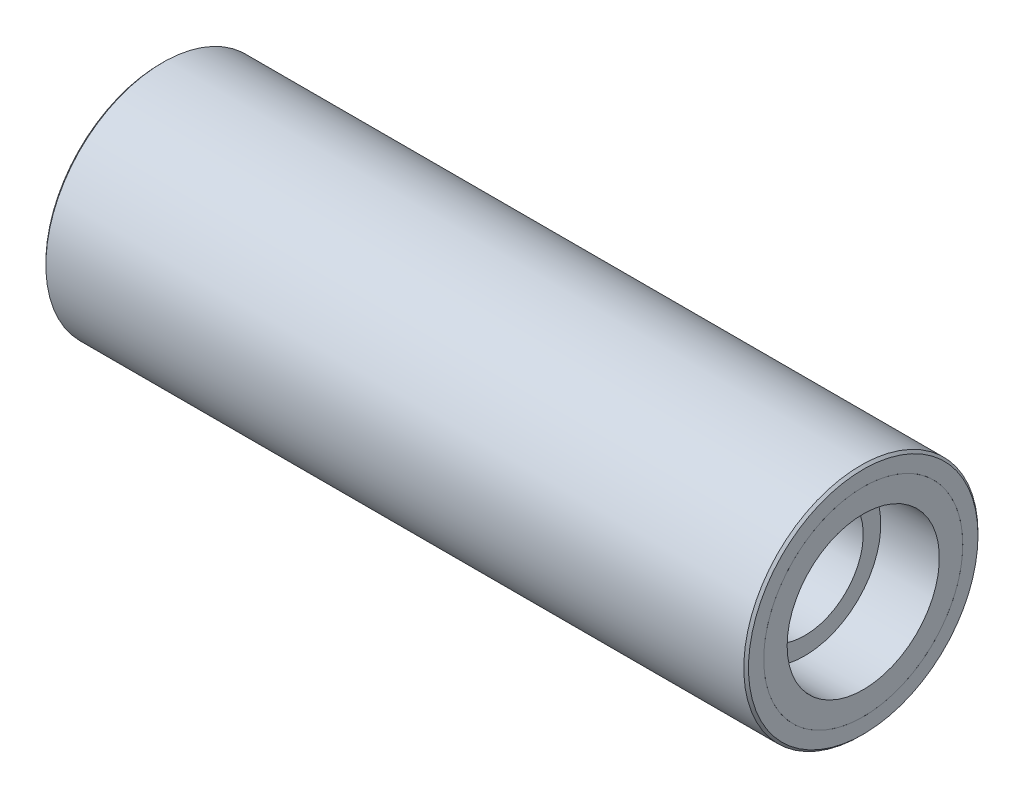
SolidWorks part; units mm, degrees
ref_plane "Front Plane" through (0, 0, 0) normal (0, 0, 1) x (1, 0, 0)
ref_plane "Top Plane" through (0, 0, 0) normal (0, 1, 0) x (1, 0, 0)
ref_plane "Right Plane" through (0, 0, 0) normal (1, 0, 0) x (0, 0, -1)
sketch "Sketch1" plane through (0, 0, 0) normal (0, 0, 1) x (1, 0, 0)
  line L0 (0, 0) -> (158.1254, 0) construction
  line L1 (0, 8.5) -> (60, 8.5)
  line L2 (60, 8.5) -> (60, 6.5)
  line L3 (60, 6.5) -> (55, 6.5)
  line L4 (55, 6.5) -> (55, 5)
  line L5 (55, 5) -> (5, 5)
  line L6 (5, 5) -> (5, 6.5)
  line L7 (5, 6.5) -> (0, 6.5)
  line L8 (0, 6.5) -> (0, 8.5)
  dimension "D1" = 60
  dimension "D2" = 10
  dimension "D3" = 13
  dimension "D4" = 5
  dimension "D5" = 17
revolve "Revolve1" add sketch "Sketch1" angle 360 about L0
sketch "Sketch2" plane through (60, 0, 0) normal (1, 0, 0) x (0, 0, -1)
  circle A0 centre (0, 0) radius 8.5
  circle A1 centre (0, 0) radius 10
  circle A2 centre (0, 0) radius 8.5 construction
  dimension "D1" = 20
extrude "Boss-Extrude1" add sketch "Sketch2" against normal up to surface (60 mm away) separate body up to face at (0, 0, 6.5)
chamfer "Chamfer1" distance 0.2 angle 45 2 edges at (0, 0, -10) (60, 0, -10)
